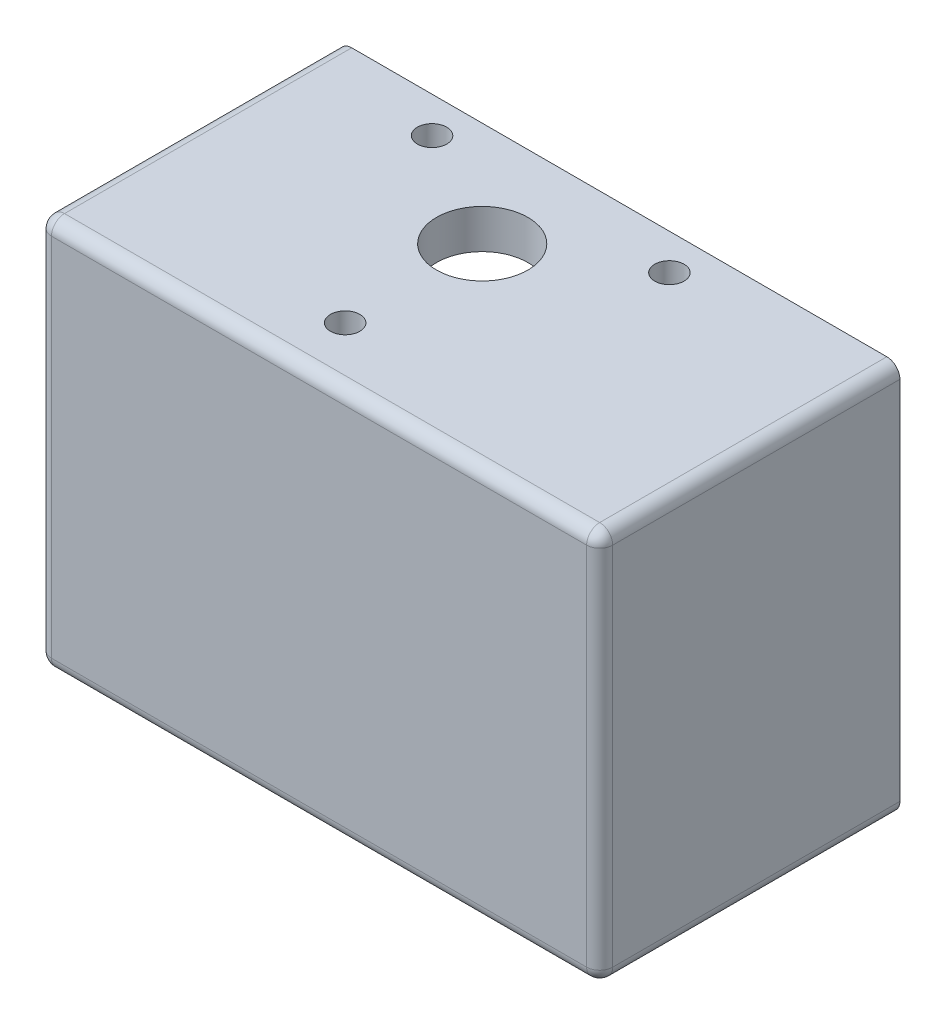
from build123d import *

# Parameters (mm, degrees)
SKETCH_1_W             = 86
SKETCH_1_H             = 60
EXTRUDE_1_DEPTH        = 46
SKETCH_2_W             = 74
SKETCH_2_H             = 48
CUT_EXTRUDE_1_DEPTH    = 41
FILLET_1_R             = 5
SKETCH_3_R             = 7
CUT_EXTRUDE_3_DEPTH    = 7
CUT_EXTRUDE_START      = -7
SKETCH_4_R             = 7
SKETCH_4_R_2           = 2.25
CUT_EXTRUDE_4_DEPTH    = 7
SKETCH_5_R             = 8.5
CUT_EXTRUDE_5_DEPTH    = 7
HOLE_WIZARD_M3_2_D     = 2.5
HOLE_WIZARD_M3_2_DEPTH = 8.5
HOLE_WIZARD_M3_2_TIP   = 0.751075774
HOLE_WIZARD_M3_3_D     = 2.5
HOLE_WIZARD_M3_3_DEPTH = 8.5
HOLE_WIZARD_M3_3_TIP   = 0.751075774
FILLET_2_R             = 2


with BuildPart() as part:
    # 草图1 → 凸台-拉伸1 (new body)
    with BuildSketch(Plane.XY):
        Rectangle(SKETCH_1_W, SKETCH_1_H)
    extrude(amount=EXTRUDE_1_DEPTH)

    # 草图2 → 切除-拉伸1 (cut)
    with BuildSketch(Plane(origin=(0, 0, 0), x_dir=(-1, 0, 0), z_dir=(0, 0, -1))):
        Rectangle(SKETCH_2_W, SKETCH_2_H)
    extrude(amount=-CUT_EXTRUDE_1_DEPTH, mode=Mode.SUBTRACT)

    # 圆角1
    fillet_1_edges = [part.edges().sort_by_distance(p)[0] for p in [
        (-37, -24, 20.5),
        (37, -24, 20.5),
        (37, 24, 20.5),
        (-37, 24, 20.5),
    ]]
    fillet(fillet_1_edges, radius=FILLET_1_R)

    # 草图3 → 切除-拉伸3 (cut)
    with BuildSketch(Plane.XZ.offset(30)):
        with Locations(Location((-5, 16, 0), (0, 0, 270))):
            Circle(SKETCH_3_R)
        with BuildLine():
            Line((25, 11.75), (29, 11.75))
            ThreePointArc((29, 11.75), (31.75, 9), (29, 6.25))
            Line((29, 6.25), (25, 6.25))
            ThreePointArc((25, 6.25), (22.25, 9), (25, 11.75))
        make_face()
        with BuildLine():
            Line((25, 33.75), (29, 33.75))
            ThreePointArc((29, 33.75), (31.75, 31), (29, 28.25))
            Line((29, 28.25), (25, 28.25))
            ThreePointArc((25, 28.25), (22.25, 31), (25, 33.75))
        make_face()
        with BuildLine():
            Line((-29, 33.75), (-25, 33.75))
            ThreePointArc((-25, 33.75), (-22.25, 31), (-25, 28.25))
            Line((-25, 28.25), (-29, 28.25))
            ThreePointArc((-29, 28.25), (-31.75, 31), (-29, 33.75))
        make_face()
        with BuildLine():
            Line((-29, 11.75), (-25, 11.75))
            ThreePointArc((-25, 11.75), (-22.25, 9), (-25, 6.25))
            Line((-25, 6.25), (-29, 6.25))
            ThreePointArc((-29, 6.25), (-31.75, 9), (-29, 11.75))
        make_face()
    extrude(amount=-CUT_EXTRUDE_3_DEPTH, mode=Mode.SUBTRACT)

    # 草图4 → 切除-拉伸4 (cut)
    with BuildSketch(Plane(origin=(0, 30, 0), x_dir=(1, 0, 0), z_dir=(0, 1, 0)).offset(CUT_EXTRUDE_START)):
        with Locations(Location((-5, -16, 0), (0, 0, 90))):
            Circle(SKETCH_4_R)
        with Locations(Location((13.186533479, -5.5, 0), (0, 0, 270))):
            Circle(SKETCH_4_R_2)
        with Locations(Location((-5, -37, 0), (0, 0, 270))):
            Circle(SKETCH_4_R_2)
        with Locations(Location((-23.186533479, -5.5, 0), (0, 0, 270))):
            Circle(SKETCH_4_R_2)
    extrude(amount=CUT_EXTRUDE_4_DEPTH, mode=Mode.SUBTRACT)

    # 草图5 → 切除-拉伸5 (cut)
    with BuildSketch(Plane.ZY.offset(43)):
        with Locations(Location((16, 0, 0), (0, 0, 270))):
            Circle(SKETCH_5_R)
    extrude(amount=-CUT_EXTRUDE_5_DEPTH, mode=Mode.SUBTRACT)

    # M3 螺纹孔2
    with Locations(Plane(origin=(-43, 0, 29.5), x_dir=(0, -1, 0), z_dir=(-1, 0, 0))):
        with Locations((0, 0), (11.691342951, -20.25), (-11.691342951, -20.25)):
            Hole(HOLE_WIZARD_M3_2_D / 2, depth=HOLE_WIZARD_M3_2_DEPTH)
            with Locations((0, 0, -(HOLE_WIZARD_M3_2_DEPTH + HOLE_WIZARD_M3_2_TIP / 2))):  # 118° drill point
                Cone(0, HOLE_WIZARD_M3_2_D / 2, HOLE_WIZARD_M3_2_TIP, mode=Mode.SUBTRACT)

    # M3 螺纹孔3
    with Locations(Plane(origin=(39.5, 25, 0), x_dir=(-1, 0, 0), z_dir=(0, 0, -1))):
        with Locations((0, 0), (79, 0), (79, -50), (0, -50)):
            Hole(HOLE_WIZARD_M3_3_D / 2, depth=HOLE_WIZARD_M3_3_DEPTH)
            with Locations((0, 0, -(HOLE_WIZARD_M3_3_DEPTH + HOLE_WIZARD_M3_3_TIP / 2))):  # 118° drill point
                Cone(0, HOLE_WIZARD_M3_3_D / 2, HOLE_WIZARD_M3_3_TIP, mode=Mode.SUBTRACT)

    # 圆角2
    fillet_2_edges = [part.edges().sort_by_distance(p)[0] for p in [
        (-43, 0, 46),
        (0, -30, 46),
        (43, 0, 46),
        (0, 30, 46),
        (43, -30, 23),
        (-43, -30, 23),
        (-43, 30, 23),
        (43, 30, 23),
    ]]
    fillet(fillet_2_edges, radius=FILLET_2_R)


solid = part.part
